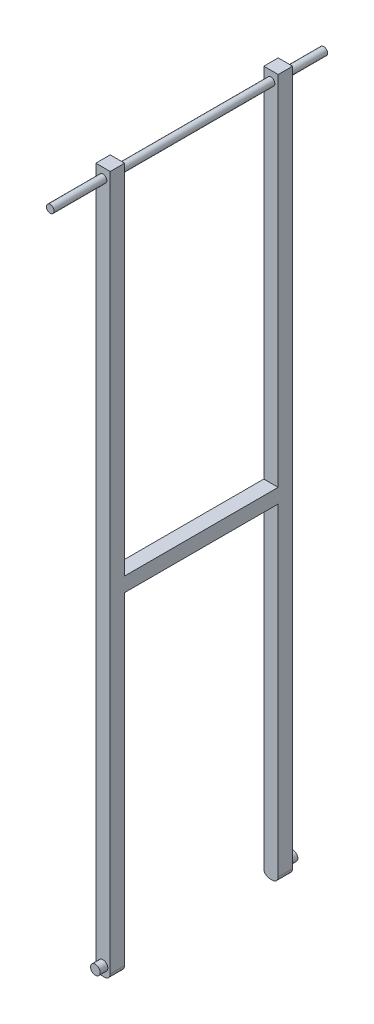
SolidWorks part; units mm, degrees
ref_plane "Front Plane" through (0, 0, 0) normal (0, 0, 1) x (1, 0, 0)
ref_plane "Top Plane" through (0, 0, 0) normal (0, 1, 0) x (1, 0, 0)
ref_plane "Right Plane" through (0, 0, 0) normal (1, 0, 0) x (0, 0, -1)
other "Configuration Table"
sketch "Sketch1" plane through (0, 0, 0) normal (0, 1, 0) x (1, 0, 0)
  line L1 (-7.5, 7.5) -> (7.5, 7.5)
  line L2 (-7.5, 7.5) -> (-7.5, -7.5)
  line L3 (-7.5, -7.5) -> (7.5, -7.5)
  line L4 (7.5, 7.5) -> (7.5, -7.5)
  line L5 (-7.5, 7.5) -> (7.5, -7.5) construction
  line L6 (-7.5, -7.5) -> (7.5, 7.5) construction
  point P0 (0, 0)
  dimension "D1" = 15
  dimension "D2" = 15
extrude "Boss-Extrude1" add sketch "Sketch1" along normal blind 730
sketch "Sketch2" plane through (0, 0, -7.5) normal (0, 0, -1) x (-1, 0, 0)
  circle A0 centre (0, 10) radius 5
  dimension "D1" = 10
  dimension "D2" = 10
extrude "Boss-Extrude2" add sketch "Sketch2" along normal blind 8
sketch "Sketch4" plane through (0, 0, 7.5) normal (0, 0, 1) x (1, 0, 0)
  line L0 (7.5, 730) -> (7.5, 0) construction
  line L1 (-7.5, 357.5) -> (7.5, 357.5)
  line L2 (-7.5, 357.5) -> (-7.5, 342.5)
  line L3 (-7.5, 342.5) -> (7.5, 342.5)
  line L4 (7.5, 357.5) -> (7.5, 342.5)
  line L5 (-7.5, 357.5) -> (7.5, 342.5) construction
  line L6 (-7.5, 342.5) -> (7.5, 357.5) construction
  line L7 (-7.5, 730) -> (7.5, 730) construction
  point P0 (0, 350)
  dimension "D1" = 15
  dimension "D2" = 15
  dimension "D3" = 350
  dimension "D4" = 380
extrude "Boss-Extrude3" add sketch "Sketch4" along normal blind 160
sketch "Sketch5" plane through (0, 0, 167.5) normal (0, 0, 1) x (1, 0, 0)
  line L0 (-7.5, 730) -> (-7.5, 357.5) construction
  line L1 (-7.5, 730) -> (7.5, 730)
  line L2 (-7.5, 730) -> (-7.5, 0)
  line L3 (-7.5, 0) -> (7.5, 0)
  line L4 (7.5, 730) -> (7.5, 0)
  line L5 (-7.5, 730) -> (7.5, 0) construction
  line L6 (-7.5, 0) -> (7.5, 730) construction
  point P0 (0, 365)
extrude "Boss-Extrude4" add sketch "Sketch5" along normal blind 15
sketch "Sketch6" plane through (0, 0, 182.5) normal (0, 0, 1) x (1, 0, 0)
  circle A0 centre (0, 10) radius 5
  dimension "D1" = 10
  dimension "D2" = 10
extrude "Boss-Extrude5" add sketch "Sketch6" along normal blind 8
fillet "Fillet1" radius 6 4 edges at (-7.5, 0, 175) (7.5, 0, 175) (-7.5, 0, 0) (7.5, 0, 0)
sketch "Sketch7" plane through (0, 0, 7.5) normal (0, 0, 1) x (1, 0, 0)
  line L0 (-7.5, 730) -> (-7.5, 6) construction
  line L1 (7.5, 730) -> (-7.5, 730) construction
  circle A0 centre (0, 720) radius 4
  dimension "D2" = 8
  dimension "D1" = 7.5
  dimension "D3" = 10
extrude "Boss-Extrude6" add sketch "Sketch7" along normal blind 230 and the other way blind 55
